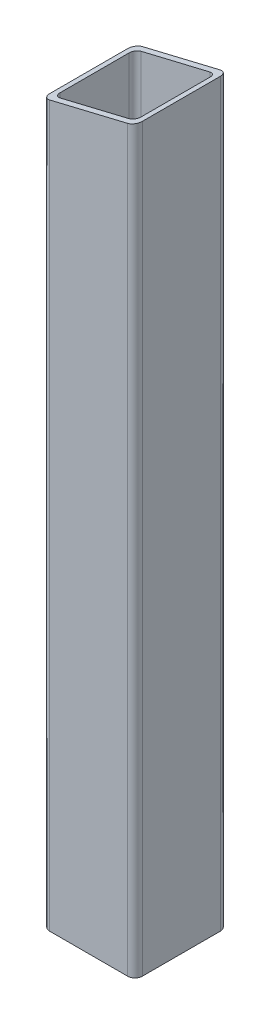
from build123d import *

# Parameters (mm, degrees)
BOSS_EXTRUDE1_DEPTH = 400
CUT_EXTRUDE1_REACH  = 426.264


with BuildPart() as part:
    # Sketch2 → Boss-Extrude1 (new, symmetric)
    with BuildSketch(Plane(origin=(0, 0, 0), x_dir=(1, 0, 0), z_dir=(0, 1, 0))):
        with BuildLine():
            Line((7.875, -1.525), (92.125, -1.525))
            ThreePointArc((92.125, -1.525), (97.693465902, 0.781534098), (100, 6.35))
            Line((100, 6.35), (100, 90.6))
            ThreePointArc((100, 90.6), (97.693465902, 96.168465902), (92.125, 98.475))
            Line((92.125, 98.475), (7.875, 98.475))
            ThreePointArc((7.875, 98.475), (2.306534098, 96.168465902), (0, 90.6))
            Line((0, 90.6), (0, 6.35))
            ThreePointArc((0, 6.35), (2.306534098, 0.781534098), (7.875, -1.525))
        make_face()
        with BuildLine():
            Line((12.6, 4.775), (87.4, 4.775))
            ThreePointArc((87.4, 4.775), (91.854772721, 6.620227279), (93.7, 11.075))
            Line((93.7, 11.075), (93.7, 85.875))
            ThreePointArc((93.7, 85.875), (91.854772721, 90.329772721), (87.4, 92.175))
            Line((87.4, 92.175), (12.6, 92.175))
            ThreePointArc((12.6, 92.175), (8.145227279, 90.329772721), (6.3, 85.875))
            Line((6.3, 85.875), (6.3, 11.075))
            ThreePointArc((6.3, 11.075), (8.145227279, 6.620227279), (12.6, 4.775))
        make_face(mode=Mode.SUBTRACT)
    extrude(amount=BOSS_EXTRUDE1_DEPTH, both=True)

    # Sketch4 → Cut-Extrude1 (cut, up to next)
    with BuildSketch(Plane.XY.offset(1.525), mode=Mode.PRIVATE) as cut_extrude1_sk1:
        Polygon((100, 400), (0, 376), (0, 400), align=None)
    cut_extrude1_tool1 = extrude(cut_extrude1_sk1.sketch, amount=-CUT_EXTRUDE1_REACH, mode=Mode.PRIVATE) & part.part
    add(cut_extrude1_tool1.solids().sort_by_distance((33.333333, 392, 1.525))[0], mode=Mode.SUBTRACT)


solid = part.part
